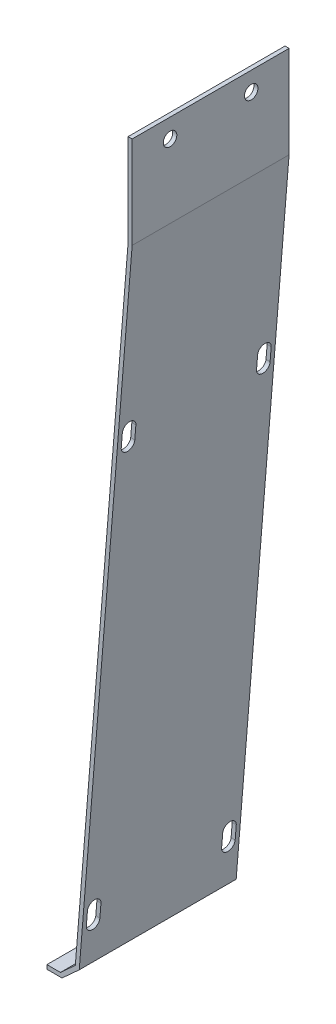
from build123d import *

# Parameters (mm, degrees)
EXTRUDE_THIN2_DEPTH = 58
SKETCH2_R           = 2.5
CUT_EXTRUDE1_DEPTH  = 10
CUT_EXTRUDE2_DEPTH  = 10


with BuildPart() as part:
    # Sketch1 → Extrude-Thin2 (new body)
    with BuildSketch(Plane.XY):
        Polygon((0, 0), (0, -34), (-19.5, -275), (-25, -280), (-30, -280), (-30, -281.5), (-24.420089688, -281.5), (-18.0526616, -275.711429011), (1.5, -34.060585647), (1.5, 0), align=None)
    extrude(amount=EXTRUDE_THIN2_DEPTH)

    # Sketch2 → Cut-Extrude1 (cut)
    with BuildSketch(Plane(origin=(1.5, 0, 0), x_dir=(0, 0, -1), z_dir=(1, 0, 0))):
        with Locations(Location((-14, -7, 0), (0, 0, 90))):
            Circle(SKETCH2_R)
        with Locations(Location((-44, -7, 0), (0, 0, 90))):
            Circle(SKETCH2_R)
    extrude(amount=-CUT_EXTRUDE1_DEPTH, mode=Mode.SUBTRACT)

    # Sketch3 → Cut-Extrude2 (cut)
    with BuildSketch(Plane(origin=(4.228257559, -0.342120425, 0), x_dir=(0, 0, -1), z_dir=(0.9967425402733565, -0.08064929267772025, 0))):
        with BuildLine():
            Line((-51.5, -97.379026061), (-51.5, -102.379026061))
            ThreePointArc((-51.5, -102.379026061), (-54, -104.879026061), (-56.5, -102.379026061))
            Line((-56.5, -102.379026061), (-56.5, -97.379026061))
            ThreePointArc((-56.5, -97.379026061), (-54, -94.879026061), (-51.5, -97.379026061))
        make_face()
        with BuildLine():
            Line((-51.5, -262.379026061), (-51.5, -257.379026061))
            ThreePointArc((-51.5, -257.379026061), (-54, -254.879026061), (-56.5, -257.379026061))
            Line((-56.5, -257.379026061), (-56.5, -262.379026061))
            ThreePointArc((-56.5, -262.379026061), (-54, -264.879026061), (-51.5, -262.379026061))
        make_face()
    cut_extrude2 = extrude(amount=-CUT_EXTRUDE2_DEPTH, mode=Mode.SUBTRACT)

    # Mirror1: Cut-Extrude2 across plane
    add(cut_extrude2.mirror(Plane.XY.offset(29)), mode=Mode.SUBTRACT)


solid = part.part
